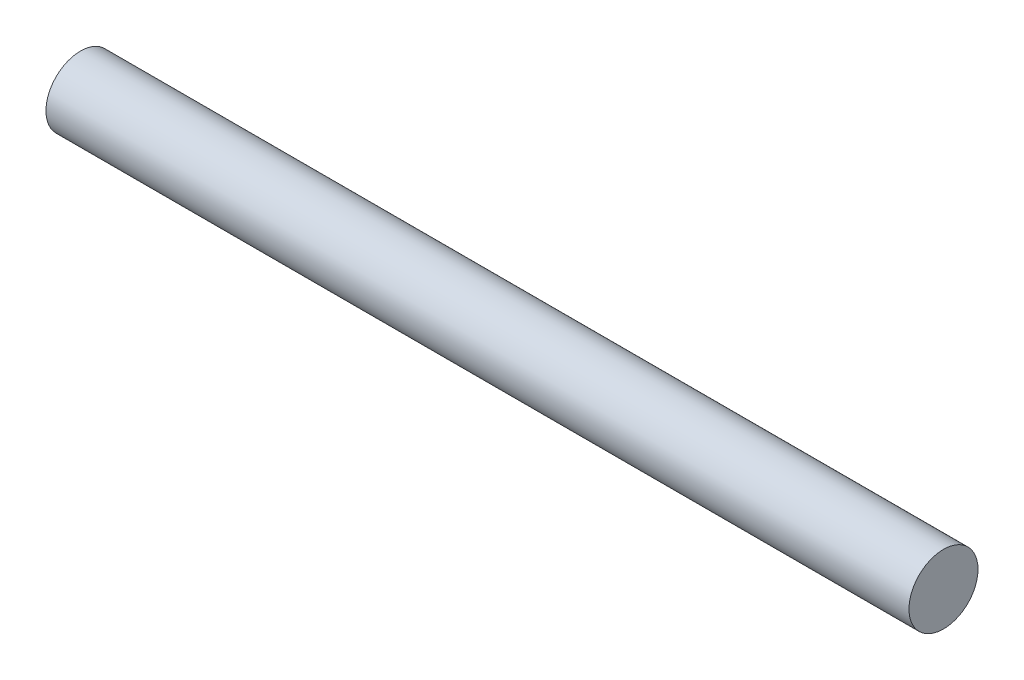
from build123d import *

# Parameters (mm, degrees)
SKETCH1_R    = 20
LENGTH_DEPTH = 500


with BuildPart() as part:
    # Sketch1 → Length (new body)
    with BuildSketch(Plane(origin=(0, 0, 0), x_dir=(0, 0, -1), z_dir=(1, 0, 0))):
        Circle(SKETCH1_R)
    extrude(amount=LENGTH_DEPTH)


solid = part.part
